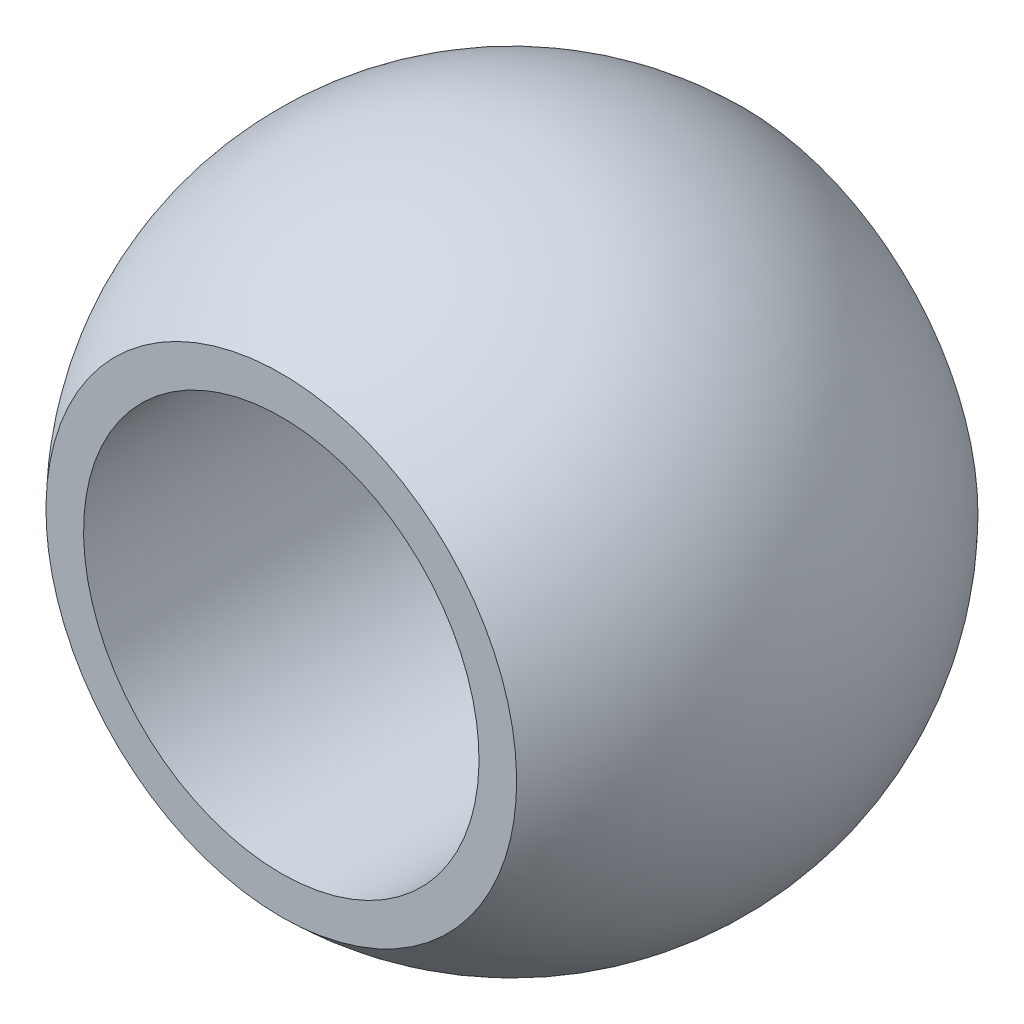
from build123d import *

# Parameters (mm, degrees)
SKETCH_2_R           = 30
CUT_EXTRUDE_1_DEPTH  = 50
SKETCH_3_OUTSIDE_W   = 136.642
SKETCH_3_OUTSIDE_H   = 136.642
SKETCH_3_OUTSIDE_W_2 = 70
SKETCH_3_OUTSIDE_H_2 = 120
CUT_EXTRUDE_2_DEPTH  = 50


with BuildPart() as part:
    # 草图1 → 旋转1 (revolve)
    with BuildSketch(Plane.XY):
        with BuildLine():
            Line((0, 50), (0, -50))
            ThreePointArc((0, -50), (50, 0), (0, 50))
        make_face()
    revolve(axis=Axis((0, 50, 0), (0, -1, 0)))

    # 草图2 → 切除-拉伸1 (cut, symmetric)
    with BuildSketch(Plane.XY):
        with Locations(Location((0, 0, 0), (0, 0, 180))):
            Circle(SKETCH_2_R)
    extrude(amount=CUT_EXTRUDE_1_DEPTH, both=True, mode=Mode.SUBTRACT)

    # 草图3 outside → 切除-拉伸2 (cut, symmetric)
    with BuildSketch(Plane(origin=(0, 0, 0), x_dir=(0, 0, -1), z_dir=(1, 0, 0))):
        Rectangle(SKETCH_3_OUTSIDE_W, SKETCH_3_OUTSIDE_H)
        Rectangle(SKETCH_3_OUTSIDE_W_2, SKETCH_3_OUTSIDE_H_2, mode=Mode.SUBTRACT)
    extrude(amount=CUT_EXTRUDE_2_DEPTH, both=True, mode=Mode.SUBTRACT)


solid = part.part
